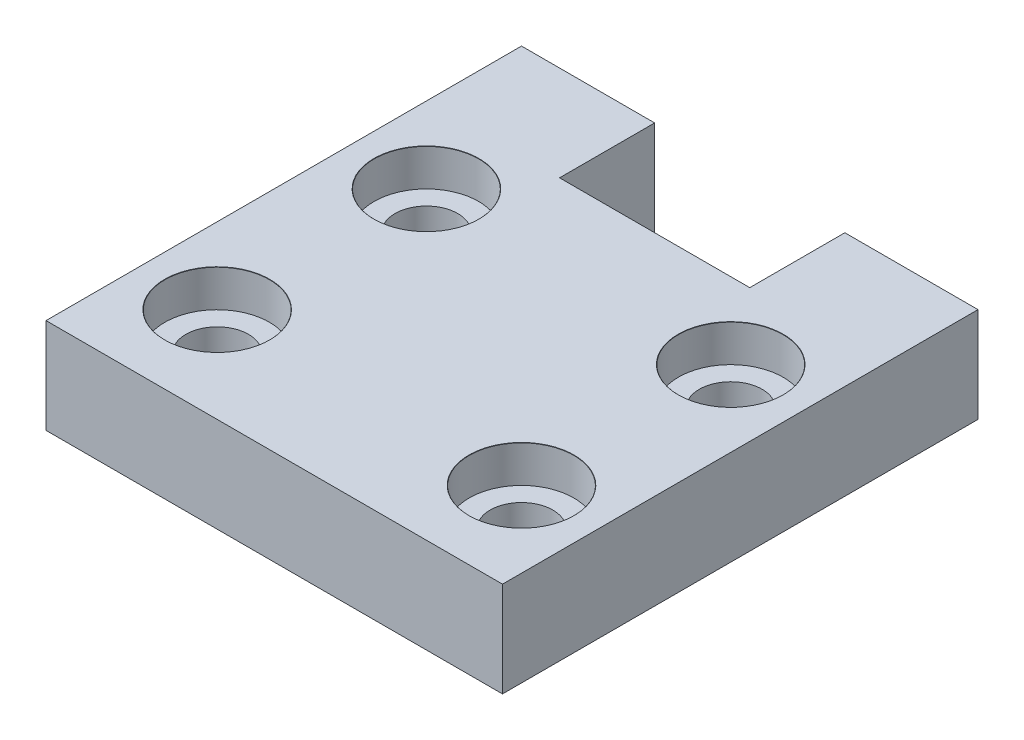
from build123d import *

# Parameters (mm, degrees)
SKETCH1_W                                  = 48
SKETCH1_H                                  = 50
BOSS_EXTRUDE1_DEPTH                        = 10
SKETCH2_W                                  = 20
SKETCH2_H                                  = 20
CUT_EXTRUDE1_DEPTH                         = 10
CBORE_FOR_M6_CHEESE_HEAD_SCREW1_AT_2_COUNT = 2
CBORE_FOR_M6_CHEESE_HEAD_SCREW1_AT_2_PITCH = 22
CBORE_FOR_M6_CHEESE_HEAD_SCREW1_AT_3_COUNT = 2
CBORE_FOR_M6_CHEESE_HEAD_SCREW1_AT_3_PITCH = 38.832975678
CBORE_FOR_M6_CHEESE_HEAD_SCREW1_AT_4_COUNT = 2
CBORE_FOR_M6_CHEESE_HEAD_SCREW1_AT_4_PITCH = 32


with BuildPart() as part:
    # Sketch1 → Boss-Extrude1 (new body)
    with BuildSketch(Plane(origin=(0, 0, 0), x_dir=(1, 0, 0), z_dir=(0, 1, 0))):
        Rectangle(SKETCH1_W, SKETCH1_H)
    extrude(amount=BOSS_EXTRUDE1_DEPTH)

    # Sketch2 → Cut-Extrude1 (cut)
    with BuildSketch(Plane(origin=(0, 10, 0), x_dir=(1, 0, 0), z_dir=(0, 1, 0))):
        with Locations((0, 25)):
            Rectangle(SKETCH2_W, SKETCH2_H)
    extrude(amount=-CUT_EXTRUDE1_DEPTH, mode=Mode.SUBTRACT)

    # Sketch4 → CBORE for M6 Cheese Head Screw1 (revolve, cut)
    with BuildSketch(Plane(origin=(-16, 10, -7), x_dir=(0, 0, 1), z_dir=(1, 0, 0))):
        Polygon((0, 0), (0, 11.982840043), (3.3, 10), (3.3, 3.9), (5.5, 3.9), (5.5, 0.025), (5.525, 0), align=None)
    cbore_for_m6_cheese_head_screw1 = revolve(axis=Axis((-16, 16.35, -7), (0, -1, 0)), mode=Mode.SUBTRACT)

    # CBORE for M6 Cheese Head Screw1 at 2: CBORE for M6 Cheese Head Screw1 ×2
    with Locations(*[(0, 0, i * CBORE_FOR_M6_CHEESE_HEAD_SCREW1_AT_2_PITCH) for i in range(1, CBORE_FOR_M6_CHEESE_HEAD_SCREW1_AT_2_COUNT)]):
        add(cbore_for_m6_cheese_head_screw1, mode=Mode.SUBTRACT)

    # CBORE for M6 Cheese Head Screw1 at 3: CBORE for M6 Cheese Head Screw1 ×2
    with Locations(*[Vector(0.8240419241993677, 0, 0.5665288228870652) * (i * CBORE_FOR_M6_CHEESE_HEAD_SCREW1_AT_3_PITCH) for i in range(1, CBORE_FOR_M6_CHEESE_HEAD_SCREW1_AT_3_COUNT)]):
        add(cbore_for_m6_cheese_head_screw1, mode=Mode.SUBTRACT)

    # CBORE for M6 Cheese Head Screw1 at 4: CBORE for M6 Cheese Head Screw1 ×2
    with Locations(*[(i * CBORE_FOR_M6_CHEESE_HEAD_SCREW1_AT_4_PITCH, 0, 0) for i in range(1, CBORE_FOR_M6_CHEESE_HEAD_SCREW1_AT_4_COUNT)]):
        add(cbore_for_m6_cheese_head_screw1, mode=Mode.SUBTRACT)


solid = part.part
